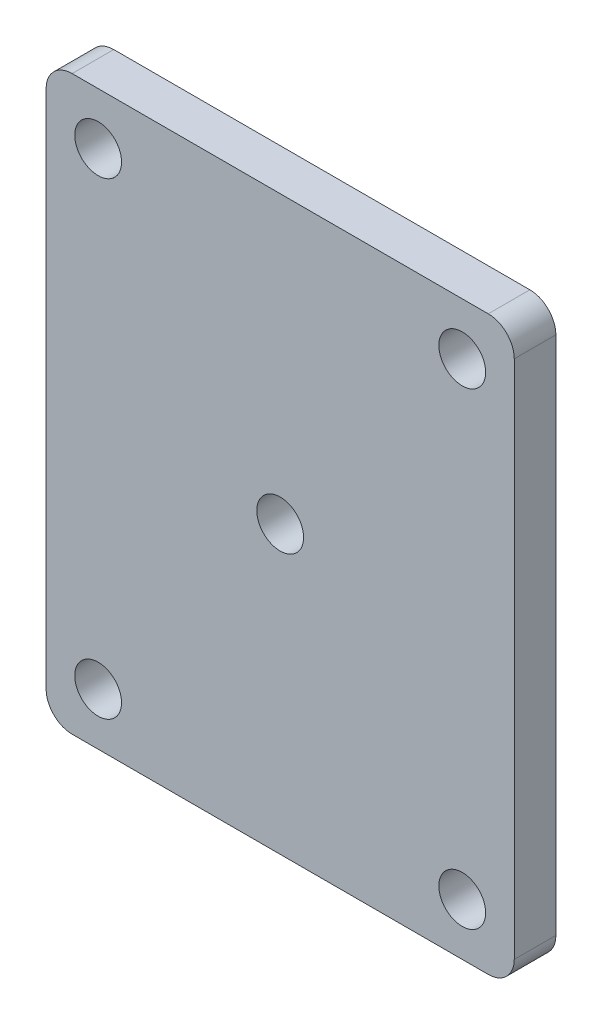
SolidWorks part; units mm, degrees
ref_plane "Front Plane" through (0, 0, 0) normal (0, 0, 1) x (1, 0, 0)
ref_plane "Top Plane" through (0, 0, 0) normal (0, 1, 0) x (1, 0, 0)
ref_plane "Right Plane" through (0, 0, 0) normal (1, 0, 0) x (0, 0, -1)
sketch "Sketch1" plane through (0, 0, 0) normal (0, 0, 1) x (1, 0, 0)
  line L0 (10, 10) -> (10, -80) construction
  line L1 (5, 20) -> (85, 20)
  line L2 (0, 15) -> (0, -85)
  line L3 (5, -90) -> (85, -90)
  line L4 (90, 15) -> (90, -85)
  line L5 (10, -80) -> (80, -80) construction
  line L6 (80, 10) -> (80, -80) construction
  line L7 (10, 10) -> (80, 10) construction
  line L8 (0, 20) -> (0, -90) construction
  line L9 (0, -90) -> (90, -90) construction
  line L10 (90, 20) -> (90, -90) construction
  line L11 (0, 20) -> (90, 20) construction
  circle A0 centre (10, 10) radius 4.5
  circle A1 centre (80, 10) radius 4.5
  circle A2 centre (10, -80) radius 4.5
  circle A3 centre (80, -80) radius 4.5
  arc A4 (0, -85) -> (5, -90) centre (5, -85) ccw
  arc A5 (90, -85) -> (85, -90) centre (85, -85) cw
  arc A6 (90, 15) -> (85, 20) centre (85, 15) ccw
  arc A7 (5, 20) -> (0, 15) centre (5, 15) ccw
  dimension "D4" = 5
  dimension "D1" = 90
  dimension "D2" = 110
  dimension "D3" = 10
extrude "Boss-Extrude1" add sketch "Sketch1" along normal blind 8
sketch "Sketch2" plane through (0, 0, 8) normal (0, 0, 1) x (1, 0, 0)
  line L0 (0, -35) -> (90, -35) construction
  line L1 (0, 15) -> (0, -85) construction
  line L2 (45, 20) -> (45, -90) construction
  line L3 (85, 20) -> (5, 20) construction
  line L4 (5, -90) -> (85, -90) construction
  line L5 (90, -85) -> (90, 15) construction
  circle A0 centre (45, -35) radius 7.2083
hole_wizard "M10x1.0 Tapped Hole1" positions "3DSketch3" profile "Sketch5" tap size "M10x1.0" standard "GB"
sketch3d "3DSketch3"
  point P0 (45, -35, 8)
sketch "Sketch5" plane through (45, -35, 8) normal (1, 0, 0) x (0, -1, 0)
  line L0 (0, 0) -> (0, 25.7039)
  line L1 (0, 25.7039) -> (4.5, 23)
  line L2 (4.5, 23) -> (4.5, 0)
  line L5 (4.5, 0) -> (0, 0)
  line L10 (0, 25.7039) -> (-4.5, 23) construction
  line L11 (0, -6.35) -> (0, 107.95) construction
  dimension "螺纹孔钻头直径" = 9
  dimension "螺纹孔钻头深度" = 23
  dimension "导头角度" = 118
cosmetic thread "Hole Thread1" parameters "D1"=8, "D2"=10
